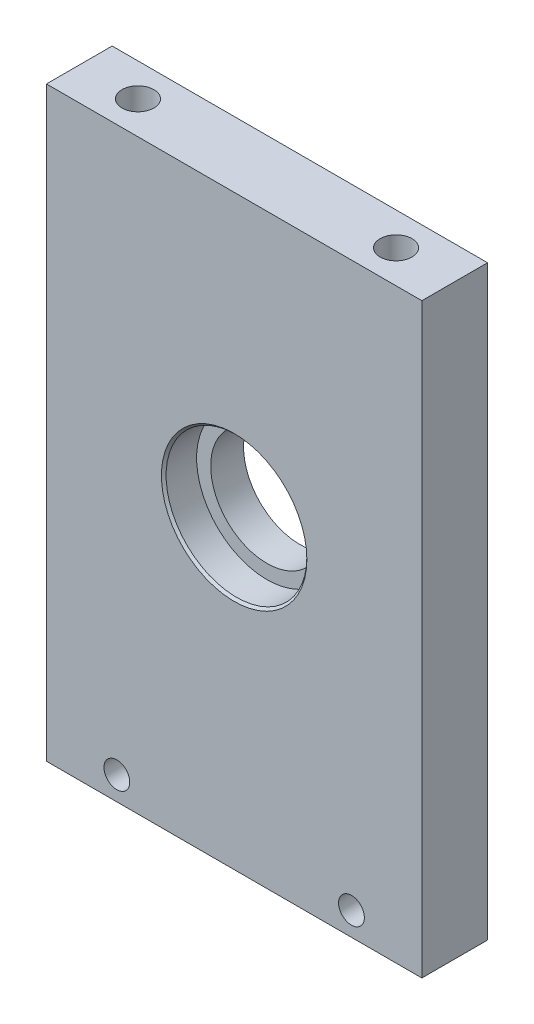
SolidWorks part; units mm, degrees
ref_plane "前视" through (0, 0, 0) normal (0, 0, 1) x (1, 0, 0)
ref_plane "上视" through (0, 0, 0) normal (0, 1, 0) x (1, 0, 0)
ref_plane "右视" through (0, 0, 0) normal (1, 0, 0) x (0, 0, -1)
sketch "草图1" plane through (0, 0, 0) normal (0, 0, 1) x (1, 0, 0)
  line L1 (0, 0) -> (80, 0)
  line L2 (0, 0) -> (0, -125)
  line L3 (0, -125) -> (80, -125)
  line L4 (80, 0) -> (80, -125)
  dimension "D1" = 80
  dimension "D2" = 125
extrude "凸台-拉伸1" add sketch "草图1" along normal blind 14
sketch "草图2" plane through (0, 0, 14) normal (0, 0, 1) x (1, 0, 0)
  line L0 (40, -60) -> (40, -125) construction
  line L1 (0, -125) -> (80, -125) construction
  circle A0 centre (40, -60) radius 15
  dimension "D1" = 30
  dimension "D2" = 65
extrude "切除-拉伸1" cut sketch "草图2" against normal blind 7
sketch "草图3" plane through (0, 0, 7) normal (0, 0, 1) x (1, 0, 0)
  circle A0 centre (40, -60) radius 12
  dimension "D1" = 24
extrude "切除-拉伸2" cut sketch "草图3" against normal through all
chamfer "倒角2" distance 0.5 angle 45 1 edges at (55, -60, 14)
hole_wizard "M8 螺纹孔1" positions "草图5" profile "草图4" tap size "M8" standard "GB"
sketch "草图5" plane through (0, 0, 0) normal (0, 1, 0) x (1, 0, 0)
  line L0 (67.5, -7) -> (12.5, -7) construction
  line L3 (40, -7) -> (40, -14) construction
  line L4 (80, -14) -> (0, -14) construction
  line L5 (0, -7) -> (31.3417, -7) construction
  line L6 (0, -14) -> (0, 0) construction
  point P0 (67.5, -7)
  point P2 (12.5, -7)
  dimension "D2" = 55
sketch "草图4" plane through (67.5, 0, 7) normal (1, 0, 0) x (0, 0, 1)
  line L0 (0, 0) -> (0, 24.2929)
  line L1 (0, 24.2929) -> (3.4, 22.25)
  line L2 (3.4, 22.25) -> (3.4, 0)
  line L5 (3.4, 0) -> (0, 0)
  line L10 (0, 24.2929) -> (-3.4, 22.25) construction
  line L11 (0, -6.35) -> (0, 107.95) construction
  dimension "螺纹孔钻头直径" = 6.8
  dimension "螺纹孔钻头深度" = 22.25
  dimension "导头角度" = 118
cosmetic thread "孔螺蚊线1" parameters "D1"=16, "D2"=8
cosmetic thread "孔螺蚊线2" parameters "D1"=16, "D2"=8
sketch "草图10" plane through (0, 0, 0) normal (0, 0, -1) x (-1, 0, 0)
  line L0 (-65, -120) -> (-15, -120) construction
  line L1 (-40, -120) -> (-40, -125) construction
  line L2 (0, -125) -> (-80, -125) construction
  circle A0 centre (-65, -120) radius 2.75
  circle A1 centre (-15, -120) radius 2.75
  dimension "D3" = 5.5
  dimension "D1" = 5
  dimension "D2" = 50
extrude "切除-拉伸3" cut sketch "草图10" against normal through all
